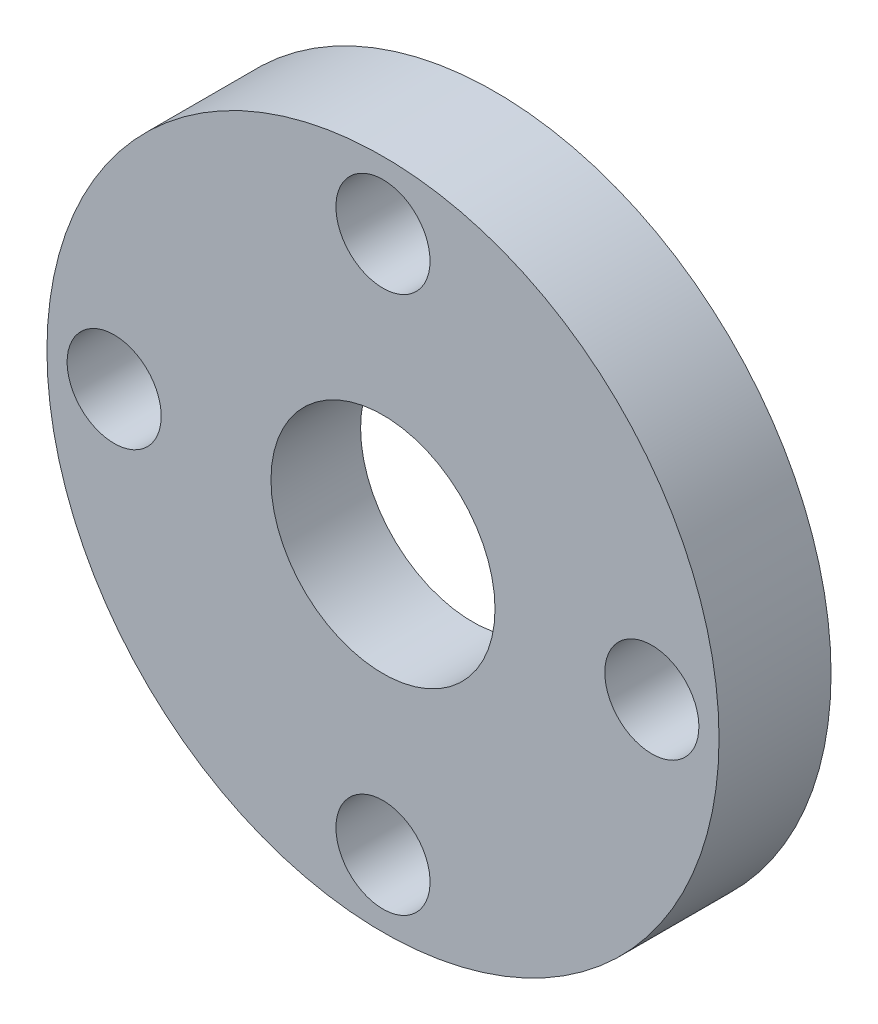
from build123d import *

# Parameters (mm, degrees)
SKETCH1_R           = 15
BOSS_EXTRUDE1_DEPTH = 5
SKETCH2_R           = 2.1
CUT_EXTRUDE1_DEPTH  = 22.794494718
CIRPATTERN1_COUNT   = 4
SKETCH3_R           = 8
CUT_EXTRUDE2_DEPTH  = 1
SKETCH4_R           = 5
CUT_EXTRUDE3_DEPTH  = 22.794494718


with BuildPart() as part:
    # Sketch1 → Boss-Extrude1 (new body)
    with BuildSketch(Plane.XY):
        Circle(SKETCH1_R)
    extrude(amount=BOSS_EXTRUDE1_DEPTH)

    # Sketch2 → Cut-Extrude1 (cut, through all)
    with BuildSketch(Plane.XY.offset(5)):
        with Locations((0, 12)):
            Circle(SKETCH2_R)
    cut_extrude1 = extrude(amount=-CUT_EXTRUDE1_DEPTH, mode=Mode.SUBTRACT)

    # CirPattern1: Cut-Extrude1 ×4 about axis
    cirpattern1_axis = Axis((0, 0, 0), (0, 0, 1))
    for i in range(1, CIRPATTERN1_COUNT):
        add(cut_extrude1.rotate(cirpattern1_axis, i * 360 / CIRPATTERN1_COUNT), mode=Mode.SUBTRACT)

    # Sketch3 → Cut-Extrude2 (cut)
    with BuildSketch(Plane(origin=(0, 0, 0), x_dir=(-1, 0, 0), z_dir=(0, 0, -1))):
        Circle(SKETCH3_R)
    extrude(amount=-CUT_EXTRUDE2_DEPTH, mode=Mode.SUBTRACT)

    # Sketch4 → Cut-Extrude3 (cut, through all)
    with BuildSketch(Plane.XY.offset(5)):
        Circle(SKETCH4_R)
    extrude(amount=-CUT_EXTRUDE3_DEPTH, mode=Mode.SUBTRACT)


solid = part.part
